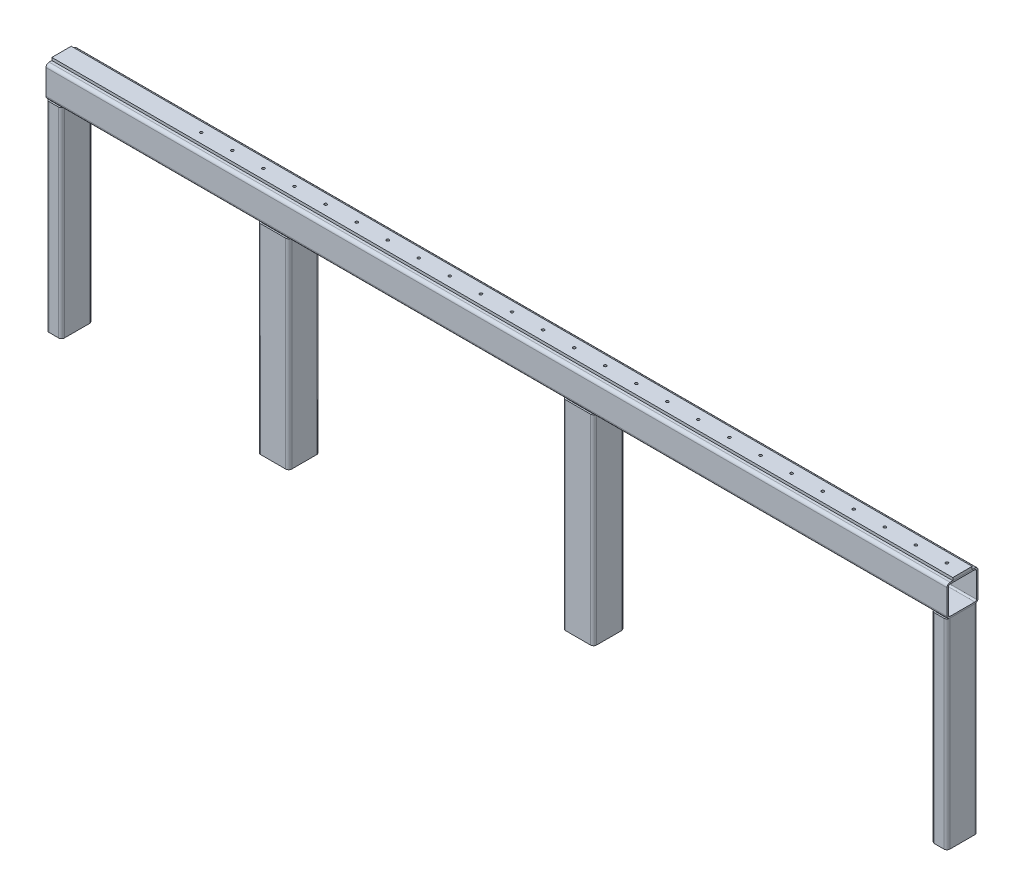
SolidWorks part; units mm, degrees
material "Q235"
ref_plane "Front" through (0, 0, 0) normal (0, 0, 1) x (1, 0, 0)
ref_plane "Top" through (0, 0, 0) normal (0, 1, 0) x (1, 0, 0)
ref_plane "Right" through (0, 0, 0) normal (1, 0, 0) x (0, 0, -1)
sketch "草图1" plane through (0, 0, 0) normal (0, 0, 1) x (1, 0, 0)
  line L0 (0, 0) -> (0, 515)
  line L1 (0, 515) -> (2280, 515)
  line L2 (2280, 515) -> (2280, 0)
  line L3 (565, 515) -> (565, 0)
  line L4 (1350, 515) -> (1350, 0)
  dimension "D1" = 2280
  dimension "D2" = 515
  dimension "D3" = 565
  dimension "D4" = 785
other "Gb／6728-1986 Rectangular Hollow Section 080 X 40 X 4(1)"
ref_plane "Plane2" through (0, 0, 0) normal (0, 1, 0) x (-1, 0, 0)
sketch "Sketch11" plane through (0, 0, 0) normal (0, 1, 0) x (-1, 0, 0)
  line L0 (-12, -36) -> (12, -36)
  line L1 (-16, -32) -> (-16, 32)
  line L2 (12, 36) -> (-12, 36)
  line L3 (16, 32) -> (16, -32)
  line L4 (-12, -40) -> (12, -40)
  line L5 (-20, -32) -> (-20, 32)
  line L6 (12, 40) -> (-12, 40)
  line L7 (20, 32) -> (20, -32)
  arc A0 (20, 32) -> (12, 40) centre (12, 32) ccw
  arc A1 (12, -40) -> (20, -32) centre (12, -32) ccw
  arc A2 (-20, -32) -> (-12, -40) centre (-12, -32) ccw
  arc A3 (-12, 40) -> (-20, 32) centre (-12, 32) ccw
  arc A4 (-12, 36) -> (-16, 32) centre (-12, 32) ccw
  arc A5 (16, 32) -> (12, 36) centre (12, 32) ccw
  arc A6 (12, -36) -> (16, -32) centre (12, -32) ccw
  arc A7 (-16, -32) -> (-12, -36) centre (-12, -32) ccw
  point P0 (0, 40)
  point P1 (20, 0)
  point P2 (0, -40)
  point P3 (-20, 0)
  point P4 (-20, 40)
  point P5 (20, 40)
  point P6 (20, -40)
  point P7 (-20, -40)
  point P8 (0, 0)
  point P33 (0, 0)
  dimension "D1" = 8
  dimension "Thickness" = 4
  dimension "V_leg" = 80
  dimension "H_leg" = 40
other "Gb／6728-1986 Square Hollow Section 080 X 80 X 4(1)"
ref_plane "Plane1" through (0, 555, 0) normal (1, 0, 0) x (0, 1, 0)
sketch "Sketch1" plane through (0, 555, 0) normal (1, 0, 0) x (0, 1, 0)
  line L0 (-32, -36) -> (32, -36)
  line L1 (-36, -32) -> (-36, 32)
  line L2 (32, 36) -> (-32, 36)
  line L3 (36, 32) -> (36, -32)
  line L4 (-32, -40) -> (32, -40)
  line L5 (-40, -32) -> (-40, 32)
  line L6 (32, 40) -> (-32, 40)
  line L7 (40, 32) -> (40, -32)
  arc A0 (40, 32) -> (32, 40) centre (32, 32) ccw
  arc A1 (32, -40) -> (40, -32) centre (32, -32) ccw
  arc A2 (-40, -32) -> (-32, -40) centre (-32, -32) ccw
  arc A3 (-32, 40) -> (-40, 32) centre (-32, 32) ccw
  arc A4 (-32, 36) -> (-36, 32) centre (-32, 32) ccw
  arc A5 (36, 32) -> (32, 36) centre (32, 32) ccw
  arc A6 (32, -36) -> (36, -32) centre (32, -32) ccw
  arc A7 (-36, -32) -> (-32, -36) centre (-32, -32) ccw
  point P0 (-40, 0)
  point P1 (40, 0)
  point P2 (0, 40)
  point P3 (0, -40)
  point P4 (0, 0)
  point P5 (-40, -40)
  point P6 (40, -40)
  point P7 (40, 40)
  point P8 (-40, 40)
  point P33 (0, 0)
  dimension "D1" = 8
  dimension "Thickness" = 4
  dimension "V_leg" = 80
other "Trim/Extend1"
other "Trim/Extend2"
sketch "Sketch2" plane through (0, 595, 0) normal (0, 1, 0) x (1, 0, 0)
  line L0 (-20, -32) -> (-20, 32) construction
  line L1 (-20, 25) -> (2300, 25)
  line L2 (-20, 25) -> (-20, -25)
  line L3 (-20, -25) -> (2300, -25)
  line L4 (2300, 25) -> (2300, -25)
  line L5 (2300, 32) -> (2300, -32) construction
  line L6 (2300, -40) -> (-20, -40) construction
  dimension "D1" = 50
  dimension "D2" = 15
extrude "Boss-Extrude1" add sketch "Sketch2" along normal blind 10 separate body
sketch "Sketch4" plane through (0, 605, 0) normal (0, 1, 0) x (1, 0, 0)
  line L0 (-20, 25) -> (-20, -25) construction
  line L1 (-20, 25) -> (2300, 25)
  line L2 (-20, 25) -> (-20, -25)
  line L3 (-20, -25) -> (2300, -25)
  line L4 (2300, 25) -> (2300, -25)
  line L5 (2300, -25) -> (2300, 25) construction
  line L6 (2300, 0) -> (2032.1771, 0) construction
  dimension "D1" = 50
extrude "Cut-Extrude1" cut sketch "Sketch4" against normal blind 3
hole_wizard "M8 Tapped Hole1" positions "Sketch5" profile "Sketch6" tap size "M8" standard "GB"
sketch "Sketch5" plane through (0, 602, 0) normal (0, 1, 0) x (1, 0, 0)
  line L0 (2300, 0) -> (2260, 0) construction
  line L1 (2300, -25) -> (2300, 25) construction
  point P0 (2260, 0)
  dimension "D1" = 40
sketch "Sketch6" plane through (2260, 602, 0) normal (1, 0, 0) x (0, 0, 1)
  line L0 (0, 0) -> (0, 21.7929)
  line L1 (0, 21.7929) -> (3.4, 19.75)
  line L2 (3.4, 19.75) -> (3.4, 0)
  line L5 (3.4, 0) -> (0, 0)
  line L10 (0, 21.7929) -> (-3.4, 19.75) construction
  line L11 (0, -6.35) -> (0, 107.95) construction
  dimension "螺纹孔钻头直径" = 6.8
  dimension "螺纹孔钻头深度" = 19.75
  dimension "导头角度" = 118
cosmetic thread "Hole Thread Line1"
pattern_linear "LPattern1" count 25 spacing 80 along (-1, 0, 0) of "M8 Tapped Hole1"
other "Square Tube 80 X 80 X 4.0(1)"
ref_plane "Plane3" through (565, 515, 0) normal (0, -1, 0) x (1, 0, 0)
sketch "Sketch12" plane through (565, 515, 0) normal (0, -1, 0) x (1, 0, 0)
  line L0 (-32, -36) -> (32, -36)
  line L1 (-36, -32) -> (-36, 32)
  line L2 (32, 36) -> (-32, 36)
  line L3 (36, 32) -> (36, -32)
  line L4 (-32, -40) -> (32, -40)
  line L5 (-40, -32) -> (-40, 32)
  line L6 (32, 40) -> (-32, 40)
  line L7 (40, 32) -> (40, -32)
  line L8 (-40, 0) -> (-36, 0) construction
  line L9 (-36, 0) -> (36, 0) construction
  line L10 (36, 0) -> (40, 0) construction
  line L12 (0, 40) -> (0, 36) construction
  line L13 (0, 36) -> (0, -36) construction
  line L14 (0, -36) -> (0, -40) construction
  arc A0 (40, 32) -> (32, 40) centre (32, 32) ccw
  arc A1 (32, -40) -> (40, -32) centre (32, -32) ccw
  arc A2 (-40, -32) -> (-32, -40) centre (-32, -32) ccw
  arc A3 (-32, 40) -> (-40, 32) centre (-32, 32) ccw
  arc A4 (-32, 36) -> (-36, 32) centre (-32, 32) ccw
  arc A5 (36, 32) -> (32, 36) centre (32, 32) ccw
  arc A6 (32, -36) -> (36, -32) centre (32, -32) ccw
  arc A7 (-36, -32) -> (-32, -36) centre (-32, -32) ccw
  point P2 (-40, 40)
  point P33 (-40, -40)
  point P34 (40, -40)
  point P36 (40, 40)
  point P37 (0, 0)
  dimension "D1" = 8
  dimension "Thickness" = 4
  dimension "V_leg" = 80
  dimension "H_leg" = 80
